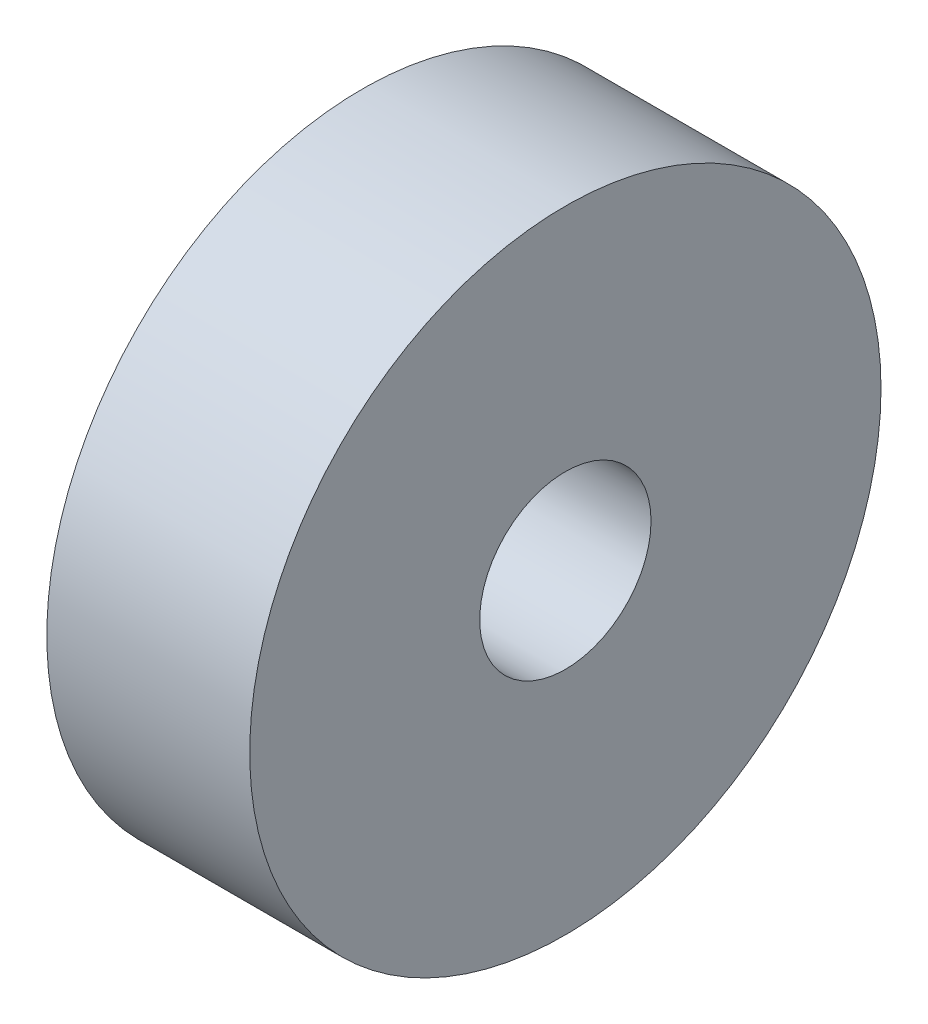
from build123d import *

# Parameters (mm, degrees)
SKETCH1_W = 90
SKETCH1_H = 102


with BuildPart() as part:
    # Sketch1 → Revolve1 (revolve)
    with BuildSketch(Plane.XY, mode=Mode.PRIVATE) as revolve1_sk:
        with Locations((0, 89)):
            Rectangle(SKETCH1_W, SKETCH1_H)
    revolve(revolve1_sk.sketch.rotate(Axis((71.901236476, 0, 0), (-1, 0, 0)), 90), axis=Axis((71.901236476, 0, 0), (-1, 0, 0)))


solid = part.part
